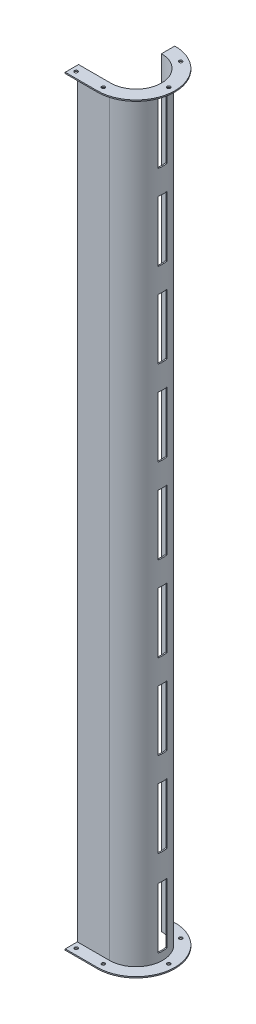
from build123d import *

# Parameters (mm, degrees)
EXTRUDE_1_DEPTH     = 1256
EXTRUDE_START       = -2
EXTRUDE_2_DEPTH     = 2
EXTRUDE_3_DEPTH     = 2
SKETCH_5_W          = 15
SKETCH_5_H          = 100
CUT_EXTRUDE_2_DEPTH = 265
SKETCH_6_R          = 2.75
CUT_EXTRUDE_3_DEPTH = 1510


with BuildPart() as part:
    # 草图1 → 凸台-拉伸1 (new body)
    with BuildSketch(Plane(origin=(0, 0, 0), x_dir=(1, 0, 0), z_dir=(0, 1, 0))):
        with BuildLine():
            Line((0, 0), (53, 0))
            ThreePointArc((53, 0), (95, 42), (53, 84))
            Line((53, 84), (53, 86))
            ThreePointArc((53, 86), (97, 42), (53, -2))
            Line((53, -2), (0, -2))
            Line((0, -2), (0, 0))
        make_face()
    extrude(amount=EXTRUDE_1_DEPTH)

    # 草图3 → 凸台-拉伸2 (add)
    with BuildSketch(Plane(origin=(0, 1256, 0), x_dir=(1, 0, 0), z_dir=(0, 1, 0)).offset(EXTRUDE_START)):
        with BuildLine():
            Line((0, 0), (53, 0))
            ThreePointArc((53, 0), (95, 42), (53, 84))
            Line((53, 84), (53, 106))
            ThreePointArc((53, 106), (117, 42), (53, -22))
            Line((53, -22), (0, -22))
            Line((0, -22), (0, 0))
        make_face()
    extrude(amount=EXTRUDE_2_DEPTH)

    # 草图4 → 凸台-拉伸3 (add)
    with BuildSketch(Plane.XZ):
        with BuildLine():
            Line((53, 0), (0, 0))
            Line((0, 0), (0, 2))
            Line((0, 2), (0, 22))
            Line((0, 22), (53, 22))
            ThreePointArc((53, 22), (117, -42), (53, -106))
            Line((53, -106), (53, -86))
            Line((53, -86), (53, -84))
            ThreePointArc((53, -84), (95, -42), (53, 0))
        make_face()
    extrude(amount=-EXTRUDE_3_DEPTH)

    # 草图5 → 切除-拉伸2 (cut)
    with BuildSketch(Plane(origin=(0, 0, 0), x_dir=(0, 0, -1), z_dir=(1, 0, 0))):
        with Locations((42.25, 65.421277154)):
            Rectangle(SKETCH_5_W, SKETCH_5_H)
        with Locations((42.25, 208)):
            Rectangle(SKETCH_5_W, SKETCH_5_H)
        with Locations((42.25, 1048)):
            Rectangle(SKETCH_5_W, SKETCH_5_H)
        with Locations((42.25, 348)):
            Rectangle(SKETCH_5_W, SKETCH_5_H)
        with Locations((42.25, 488)):
            Rectangle(SKETCH_5_W, SKETCH_5_H)
        with Locations((42.25, 628)):
            Rectangle(SKETCH_5_W, SKETCH_5_H)
        with Locations((42.25, 768)):
            Rectangle(SKETCH_5_W, SKETCH_5_H)
        with Locations((42.25, 908)):
            Rectangle(SKETCH_5_W, SKETCH_5_H)
        with Locations((42.25, 1188)):
            Rectangle(SKETCH_5_W, SKETCH_5_H)
    extrude(amount=CUT_EXTRUDE_2_DEPTH, mode=Mode.SUBTRACT)

    # 草图6 → 切除-拉伸3 (cut)
    with BuildSketch(Plane(origin=(0, 1256, 0), x_dir=(1, 0, 0), z_dir=(0, 1, 0))):
        with Locations(Location((80, 88.765371804, 0), (0, 0, 270))):
            Circle(SKETCH_6_R)
        with Locations(Location((107, 42, 0), (0, 0, 270))):
            Circle(SKETCH_6_R)
        with Locations(Location((53, -12, 0), (0, 0, 270))):
            Circle(SKETCH_6_R)
        with Locations(Location((8, -12, 0), (0, 0, 270))):
            Circle(SKETCH_6_R)
    extrude(amount=-CUT_EXTRUDE_3_DEPTH, mode=Mode.SUBTRACT)


solid = part.part
